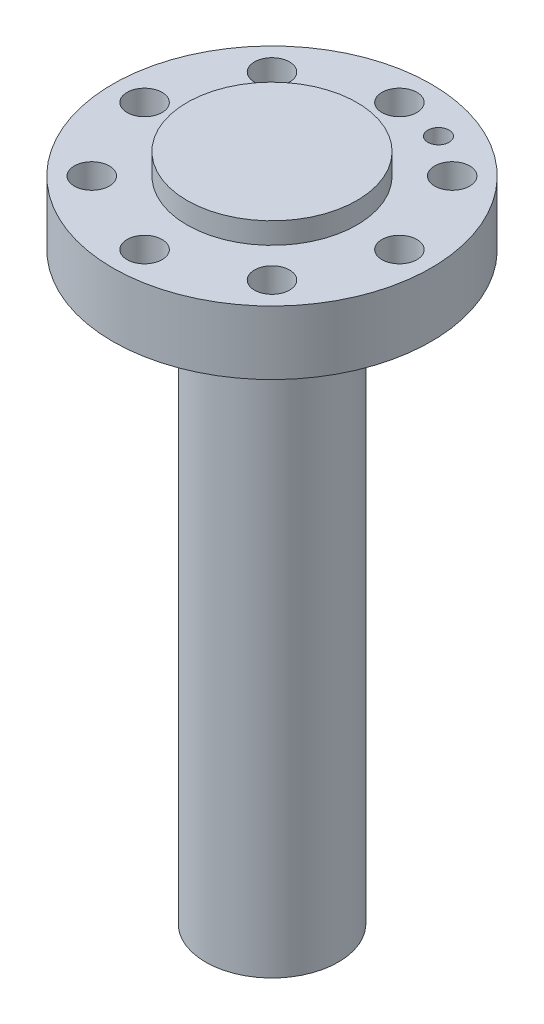
SolidWorks part; units mm, degrees
material "AL6061"
ref_plane "前视" through (0, 0, 0) normal (0, 0, 1) x (1, 0, 0)
ref_plane "上视" through (0, 0, 0) normal (0, 1, 0) x (1, 0, 0)
ref_plane "右视" through (0, 0, 0) normal (1, 0, 0) x (0, 0, -1)
sketch "草图1" plane through (0, 0, 0) normal (0, 1, 0) x (1, 0, 0)
  circle A0 centre (0, 0) radius 30
  dimension "D1" = 60
extrude "凸台-拉伸1" add sketch "草图1" along normal blind 122
sketch "草图2" plane through (0, 122, 0) normal (0, 1, 0) x (1, 0, 0)
  circle A0 centre (0, 0) radius 12.5
  dimension "D1" = 25
extrude "切除-拉伸1" cut sketch "草图2" against normal through all from offset 12 flip side to cut offset against normal yes
hole_wizard "M6 间隙孔1" positions "草图5" profile "草图6" hole size "M6" standard "ISO" end condition through all
sketch "草图5" plane through (0, 110, 0) normal (0, -1, 0) x (-1, 0, 0)
  line L0 (0, 0) -> (-24, 0) construction
  point P0 (-24, 0)
  point P7 (-16.9706, 16.9706)
  point P8 (0, 24)
  point P9 (16.9706, 16.9706)
  point P10 (24, 0)
  point P11 (16.9706, -16.9706)
  point P16 (0, -24)
  point P17 (-16.9706, -16.9706)
  dimension "D2" = 24
  dimension "D1" = 8
sketch "草图6" plane through (24, 110, 0) normal (1, 0, 0) x (0, 0, -1)
  line L0 (0, 0) -> (0, 12)
  line L1 (0, 12) -> (3.3, 12)
  line L2 (3.3, 12) -> (3.3, 0)
  line L5 (3.3, 0) -> (0, 0)
  line L11 (0, -6.35) -> (0, 107.95) construction
  dimension "通孔孔直径" = 6.6
  dimension "通孔孔深度" = 12
sketch "草图7" plane through (0, 122, 0) normal (0, 1, 0) x (1, 0, 0)
  circle A0 centre (0, 0) radius 16
  dimension "D1" = 32
extrude "凸台-拉伸3" add sketch "草图7" along normal blind 4
hole_wizard "大小mm 暗销孔0" positions "草图12" profile "草图13" hole size "Ø4.0" standard "GB" end condition through all
sketch "草图12" plane through (0, 110, 0) normal (0, -1, 0) x (-1, 0, 0)
  line L0 (0, 0) -> (-9.1844, 22.1731) construction
  line L1 (0, 0) -> (24, 0) construction
  circle A0 centre (0, 0) radius 24
  point P5 (-9.1844, 22.1731)
  dimension "D1" = 48
  dimension "D2" = 112.5
sketch "草图13" plane through (9.1844, 110, -22.1731) normal (1, 0, 0) x (0, 0, -1)
  line L0 (0, 0) -> (0, 16)
  line L1 (0, 16) -> (2, 16)
  line L2 (2, 16) -> (2, 0)
  line L5 (2, 0) -> (0, 0)
  line L11 (0, -6.35) -> (0, 107.95) construction
  dimension "通孔孔直径" = 4
  dimension "通孔孔深度" = 16
ref_plane "基准面1" through (15, 0, 0) normal (1, 0, 0) x (0, 0, -1)
hole_wizard "M6 螺纹孔1" positions "草图14" profile "草图15" tap size "M6" standard "GB"
sketch "草图14" plane through (0, 0, 0) normal (0, -1, 0) x (-1, 0, 0)
  point P0 (0, 0)
sketch "草图15" plane through (0, 0, 0) normal (1, 0, 0) x (0, 0, -1)
  line L0 (0, 0) -> (0, 16.5022)
  line L1 (0, 16.5022) -> (2.5, 15)
  line L2 (2.5, 15) -> (2.5, 0)
  line L5 (2.5, 0) -> (0, 0)
  line L10 (0, 16.5022) -> (-2.5, 15) construction
  line L11 (0, -6.35) -> (0, 107.95) construction
  dimension "螺纹孔钻头直径" = 5
  dimension "螺纹孔钻头深度" = 15
  dimension "导头角度" = 118
cosmetic thread "孔螺蚊线1" parameters "D1"=12, "D2"=6
